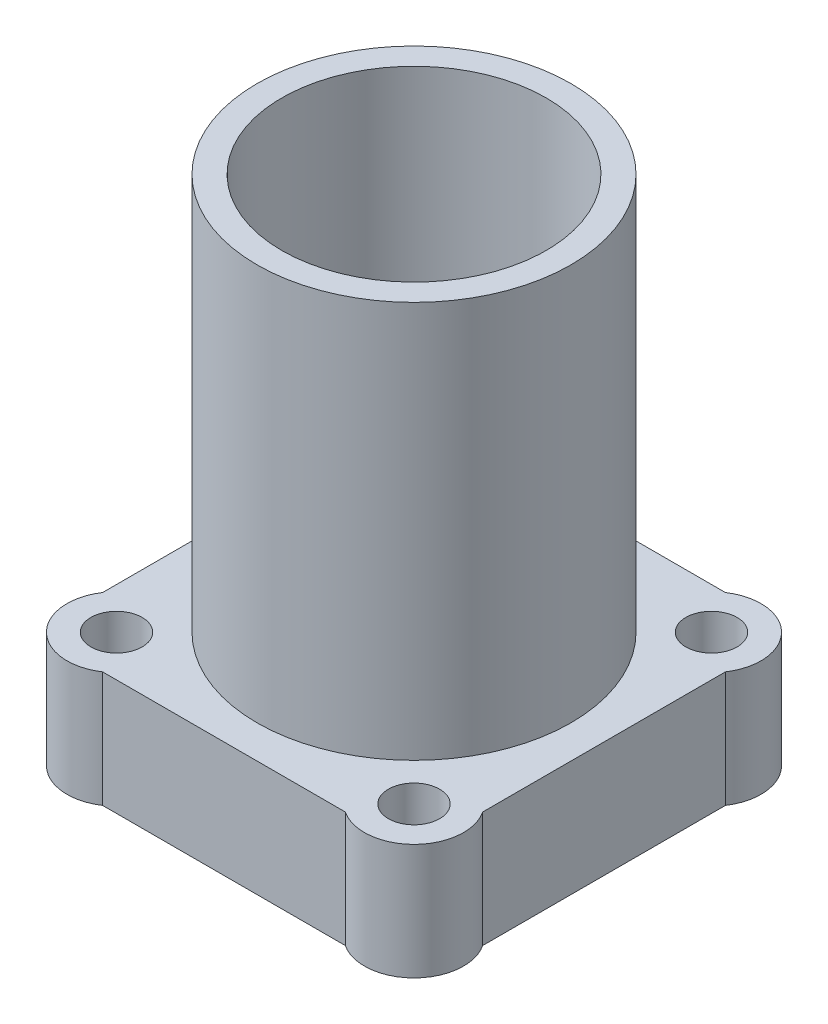
SolidWorks part; units mm, degrees
material "6061 合金"
ref_plane "前视基准面" through (0, 0, 0) normal (0, 0, 1) x (1, 0, 0)
ref_plane "上视基准面" through (0, 0, 0) normal (0, 1, 0) x (1, 0, 0)
ref_plane "右视基准面" through (0, 0, 0) normal (1, 0, 0) x (0, 0, -1)
other "Configuration Table"
sketch "草图1" plane through (0, 0, 0) normal (0, 1, 0) x (1, 0, 0)
  line L0 (-7.3417, 11.5) -> (7.3417, 11.5)
  line L1 (-9, 9) -> (9, 9) construction
  line L2 (-9, 9) -> (-9, -9) construction
  line L3 (-9, -9) -> (9, -9) construction
  line L4 (9, 9) -> (9, -9) construction
  line L5 (-9, 9) -> (9, -9) construction
  line L6 (-9, -9) -> (9, 9) construction
  line L7 (11.5, -7.3417) -> (11.5, 7.3417)
  line L9 (-11.5, 7.3417) -> (-11.5, -7.3417)
  line L10 (7.3417, -11.5) -> (-7.3417, -11.5)
  circle A0 centre (9, 9) radius 1.55
  circle A1 centre (9, -9) radius 1.55
  circle A2 centre (-9, -9) radius 1.55
  circle A3 centre (-9, 9) radius 1.55
  circle A4 centre (9, 9) radius 3
  circle A5 centre (-9, 9) radius 3
  circle A6 centre (-9, -9) radius 3
  circle A7 centre (9, -9) radius 3
  circle A8 centre (0, 0) radius 7
  point P0 (0, 0)
  dimension "D2" = 3.1
  dimension "D3" = 6
  dimension "D4" = 14
  dimension "D1" = 18
  dimension "D5" = 2.5
  dimension "D6" = 2.5
extrude "凸台-拉伸1" add sketch "草图1" along normal blind 7
sketch "草图2" plane through (0, 7, 0) normal (0, 1, 0) x (1, 0, 0)
  circle A3 centre (0, 0) radius 8
  circle A4 centre (0, 0) radius 9.5
  dimension "D1" = 16
  dimension "D2" = 1.5
extrude "凸台-拉伸2" add sketch "草图2" along normal blind 24
